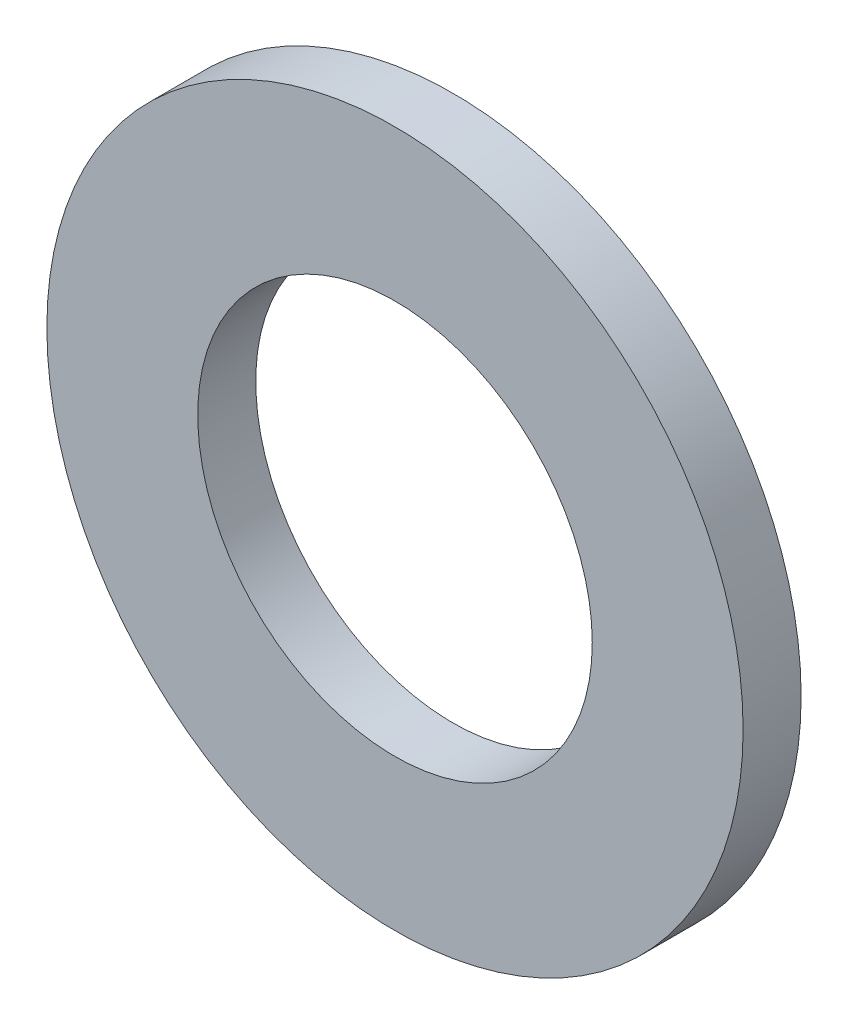
from build123d import *

# Parameters (mm, degrees)
SKETCH_1_R      = 9
SKETCH_1_R_2    = 5.1
EXTRUDE_1_DEPTH = 0.75


with BuildPart() as part:
    # 草图1 → 凸台-拉伸1 (new, symmetric)
    with BuildSketch(Plane.XY):
        Circle(SKETCH_1_R)
        Circle(SKETCH_1_R_2, mode=Mode.SUBTRACT)
    extrude(amount=EXTRUDE_1_DEPTH, both=True)


solid = part.part
